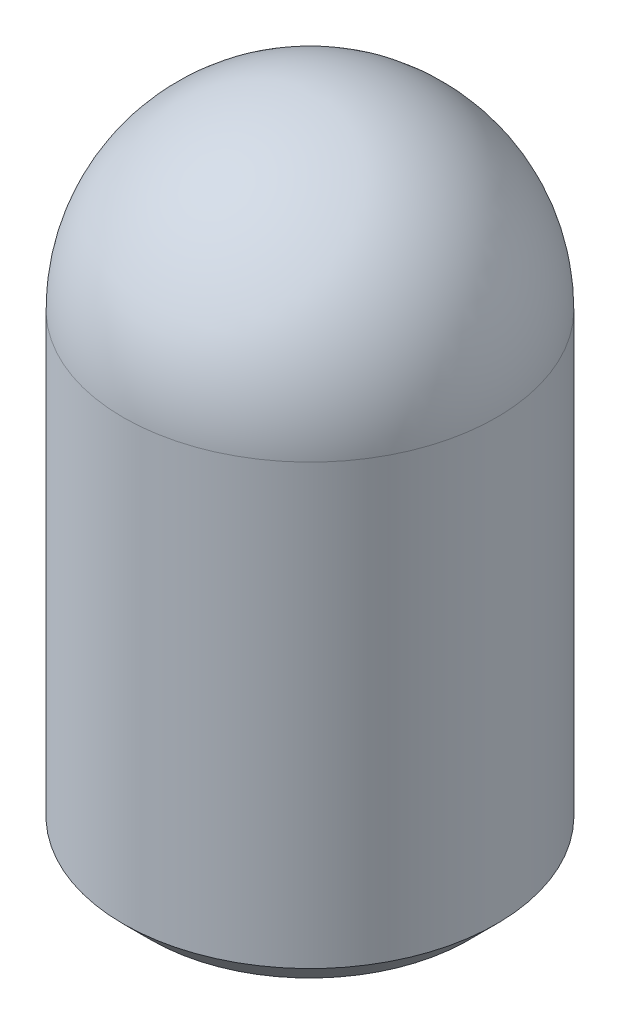
from build123d import *

# Parameters (mm, degrees)
SKETCH1_R           = 2
BOSS_EXTRUDE1_DEPTH = 2.5
DOME1_FACE_RADIUS   = 2
DOME1_HEIGHT        = 2
CHAMFER1_SIZE       = 0.3


with BuildPart() as part:
    # Sketch1 → Boss-Extrude1 (new, symmetric)
    with BuildSketch(Plane(origin=(0, 0, 0), x_dir=(1, 0, 0), z_dir=(0, 1, 0))):
        with Locations(Location((0, 0, 0), (0, 0, 270))):
            Circle(SKETCH1_R)
    extrude(amount=BOSS_EXTRUDE1_DEPTH, both=True)

    # Dome1: a dome of height H over a round flat face of radius A is a cap of a sphere of radius (A * A + H * H) / (2 * H)
    dome1_r = (DOME1_FACE_RADIUS * DOME1_FACE_RADIUS + DOME1_HEIGHT * DOME1_HEIGHT) / (2 * DOME1_HEIGHT)
    dome1_base = Plane((0, 2.5, 0), z_dir=(0, 1, 0))
    with Locations(dome1_base.offset(DOME1_HEIGHT - dome1_r)):
        dome1_ball = Sphere(dome1_r, mode=Mode.PRIVATE)
    add(split(dome1_ball, bisect_by=dome1_base, keep=Keep.TOP, mode=Mode.PRIVATE))

    # Chamfer1
    chamfer1_edges = [part.edges().sort_by_distance(p)[0] for p in [
        (0, -2.5, -2),
    ]]
    chamfer(chamfer1_edges, length=CHAMFER1_SIZE)


solid = part.part
